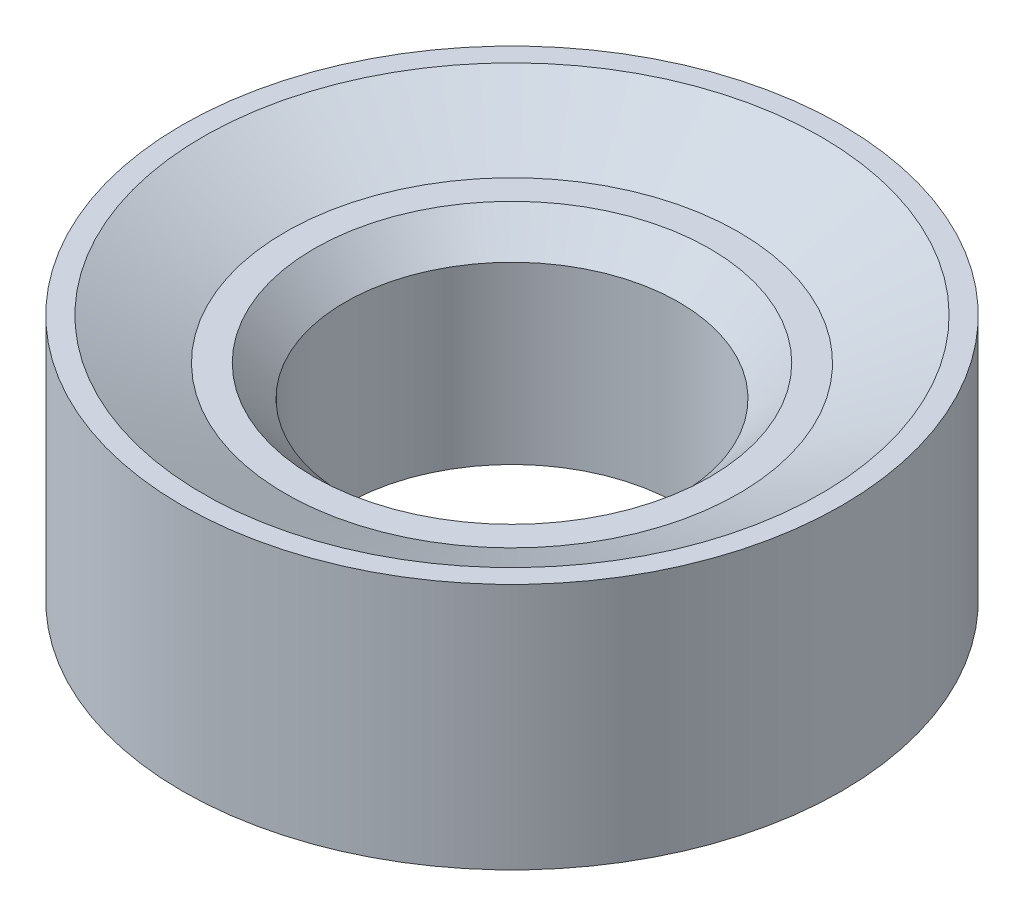
SolidWorks part; units mm, degrees
material "35#"
ref_plane "Front Plane" through (0, 0, 0) normal (0, 0, 1) x (1, 0, 0)
ref_plane "Top Plane" through (0, 0, 0) normal (0, 1, 0) x (1, 0, 0)
ref_plane "Right Plane" through (0, 0, 0) normal (1, 0, 0) x (0, 0, -1)
sketch "Sketch1" plane through (0, 0, 0) normal (0, 0, 1) x (1, 0, 0)
  line L0 (0, 0) -> (0, 30) construction
  line L1 (20, 0) -> (40, 0)
  line L2 (40, 0) -> (40, 30)
  line L3 (40, 30) -> (37.5, 30)
  line L4 (37.5, 30) -> (27.5, 25)
  line L5 (27.5, 25) -> (24, 25)
  line L7 (20, 21) -> (20, 0)
  line L8 (24, 25) -> (20, 21)
  dimension "D1" = 30
  dimension "D2" = 80
  dimension "D3" = 75
  dimension "D4" = 55
  dimension "D5" = 48
  dimension "D6" = 25
  dimension "D7" = 45
  dimension "D8" = 21
revolve "Revolve1" add sketch "Sketch1" angle 360 about L0
hole_wizard "M42X1.5 Tapped Hole1" positions "Sketch4" profile "Sketch5" tap size "M42X1.5" standard "GB"
sketch "Sketch4" plane through (0, 0, 0) normal (0, -1, 0) x (-1, 0, 0)
  point P0 (0, 0)
sketch "Sketch5" plane through (0, 0, 0) normal (1, 0, 0) x (0, 0, -1)
  line L0 (0, 0) -> (0, 100.6674)
  line L1 (0, 100.6674) -> (20.25, 88.5)
  line L2 (20.25, 88.5) -> (20.25, 0)
  line L5 (20.25, 0) -> (0, 0)
  line L10 (0, 100.6674) -> (-20.25, 88.5) construction
  line L11 (0, -6.35) -> (0, 107.95) construction
  dimension "螺纹孔钻头直径" = 40.5
  dimension "螺纹孔钻头深度" = 88.5
  dimension "导头角度" = 118
cosmetic thread "Cosmetic thread 1" parameters "D1"=84, "D2"=41.5
